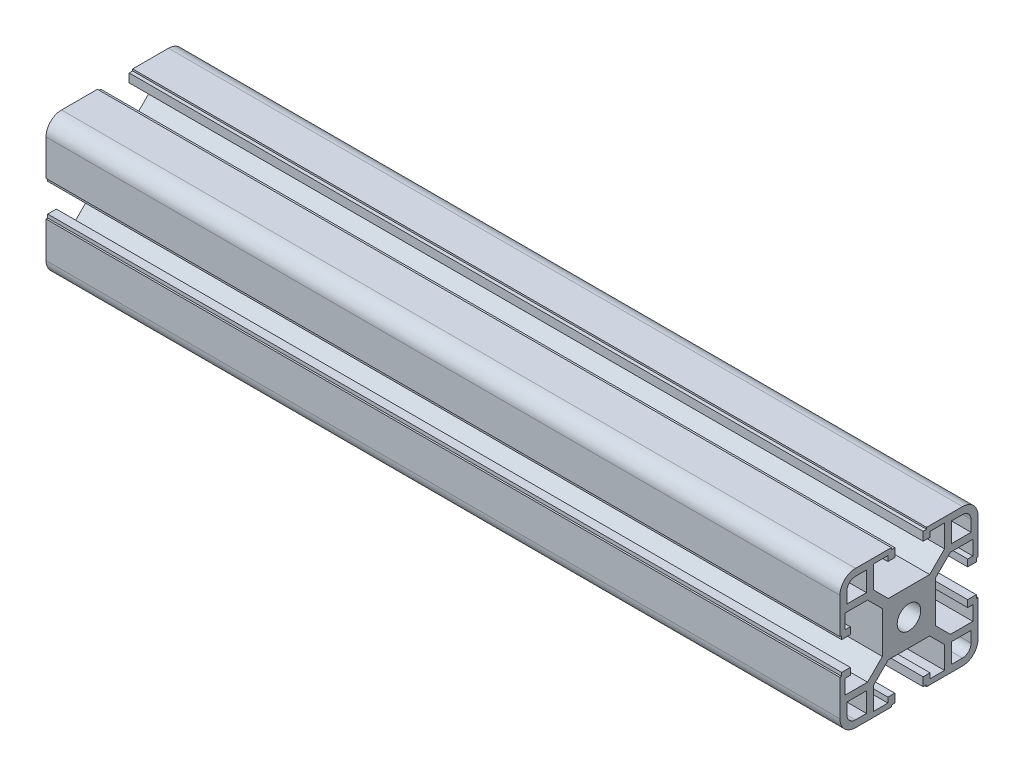
SolidWorks part; units mm, degrees
ref_plane "Front Plane" through (0, 0, 0) normal (0, 0, 1) x (1, 0, 0)
ref_plane "Top Plane" through (0, 0, 0) normal (0, 1, 0) x (1, 0, 0)
ref_plane "Right Plane" through (0, 0, 0) normal (1, 0, 0) x (0, 0, -1)
sketch "草图1" plane through (0, 0, 0) normal (0, 0, 1) x (1, 0, 0)
  line L0 (-984.975, 0) -> (-754.975, 0)
  dimension "D1" = 230
other "Aluminium profile 40 X 40B X R4.5(1)"
ref_plane "Plane1" through (-984.975, 0, 0) normal (1, 0, 0) x (0, 1, 0)
sketch "Sketch1" plane through (-984.975, 0, 0) normal (1, 0, 0) x (0, 1, 0)
  line L0 (-5.1, 20) -> (-5.1, 19.5)
  line L1 (-5.1, 19.5) -> (-4.1, 19.5)
  line L2 (-4.1, 19.5) -> (-4.1, 17)
  line L3 (-6.1, 18.5) -> (-10.3, 18.5)
  line L4 (-15.5, -20) -> (-5.1, -20)
  line L5 (-20, -15.5) -> (-20, -5.1)
  line L6 (15.5, 20) -> (5.1, 20)
  line L7 (20, 15.5) -> (20, 5.1)
  line L8 (0, 14.8756) -> (0, 0) construction
  line L9 (0, 0) -> (14.1675, 0) construction
  line L10 (-10.3, 18.5) -> (-10.3, 12)
  line L11 (-10.3, 12) -> (-6, 7.7)
  line L12 (-6, 7.7) -> (6, 7.7)
  line L13 (10.3, 12) -> (6, 7.7)
  line L14 (10.3, 18.5) -> (10.3, 12)
  line L15 (6.1, 18.5) -> (10.3, 18.5)
  line L16 (4.1, 19.5) -> (4.1, 17)
  line L17 (5.1, 19.5) -> (4.1, 19.5)
  line L18 (5.1, 20) -> (5.1, 19.5)
  line L19 (-5.1, 20) -> (-15.5, 20)
  line L20 (20, 5.1) -> (19.5, 5.1)
  line L21 (12.3, 18) -> (15.5, 18)
  line L22 (12.3, 18) -> (12.3, 12.3)
  line L23 (12.3, 12.3) -> (18, 12.3)
  line L24 (18, 15.5) -> (18, 12.3)
  line L25 (19.5, 5.1) -> (19.5, 4.1)
  line L26 (19.5, 4.1) -> (17, 4.1)
  line L27 (17, 6.1) -> (17, 4.1)
  line L28 (18.5, 6.1) -> (17, 6.1)
  line L29 (18.5, 6.1) -> (18.5, 10.3)
  line L30 (18.5, 10.3) -> (12, 10.3)
  line L31 (12, 10.3) -> (7.7, 6)
  line L32 (7.7, 6) -> (7.7, -6)
  line L33 (12, -10.3) -> (7.7, -6)
  line L34 (18.5, -10.3) -> (12, -10.3)
  line L35 (18.5, -6.1) -> (18.5, -10.3)
  line L36 (18.5, -6.1) -> (17, -6.1)
  line L37 (17, -4.1) -> (17, -6.1)
  line L38 (19.5, -4.1) -> (17, -4.1)
  line L39 (19.5, -5.1) -> (19.5, -4.1)
  line L40 (20, -5.1) -> (19.5, -5.1)
  line L41 (5.1, -20) -> (5.1, -19.5)
  line L42 (5.1, -19.5) -> (4.1, -19.5)
  line L43 (4.1, -19.5) -> (4.1, -17)
  line L44 (6.1, -17) -> (4.1, -17)
  line L45 (6.1, -18.5) -> (6.1, -17)
  line L46 (6.1, -18.5) -> (10.3, -18.5)
  line L47 (10.3, -18.5) -> (10.3, -12)
  line L48 (10.3, -12) -> (6, -7.7)
  line L49 (6, -7.7) -> (-6, -7.7)
  line L50 (-10.3, -12) -> (-6, -7.7)
  line L51 (-10.3, -18.5) -> (-10.3, -12)
  line L52 (-6.1, -18.5) -> (-10.3, -18.5)
  line L53 (-6.1, -18.5) -> (-6.1, -17)
  line L54 (-4.1, -17) -> (-6.1, -17)
  line L55 (-4.1, -19.5) -> (-4.1, -17)
  line L56 (-5.1, -19.5) -> (-4.1, -19.5)
  line L57 (-5.1, -20) -> (-5.1, -19.5)
  line L58 (-20, -5.1) -> (-19.5, -5.1)
  line L59 (5.1, -20) -> (15.5, -20)
  line L60 (-20, 5.1) -> (-20, 15.5)
  line L61 (-19.5, -5.1) -> (-19.5, -4.1)
  line L62 (-6.1, 18.5) -> (-6.1, 17)
  line L63 (-6.1, 17) -> (-4.1, 17)
  line L64 (6.1, 18.5) -> (6.1, 17)
  line L65 (4.1, 17) -> (6.1, 17)
  line L66 (-19.5, -4.1) -> (-17, -4.1)
  line L67 (-15.5, 18) -> (-12.3, 18)
  line L68 (-18, 15.5) -> (-18, 12.3)
  line L69 (-18, 12.3) -> (-12.3, 12.3)
  line L70 (-12.3, 18) -> (-12.3, 12.3)
  line L71 (-17, -6.1) -> (-17, -4.1)
  line L72 (-18.5, -6.1) -> (-17, -6.1)
  line L73 (-18.5, -6.1) -> (-18.5, -10.3)
  line L74 (-18.5, -10.3) -> (-12, -10.3)
  line L75 (-12, -10.3) -> (-7.7, -6)
  line L76 (-7.7, -6) -> (-7.7, 6)
  line L77 (-12, 10.3) -> (-7.7, 6)
  line L78 (-18.5, 10.3) -> (-12, 10.3)
  line L79 (-18.5, 6.1) -> (-18.5, 10.3)
  line L80 (-18.5, 6.1) -> (-17, 6.1)
  line L81 (-17, 4.1) -> (-17, 6.1)
  line L82 (-19.5, 4.1) -> (-17, 4.1)
  line L83 (-19.5, 5.1) -> (-19.5, 4.1)
  line L84 (-20, 5.1) -> (-19.5, 5.1)
  line L85 (20, -5.1) -> (20, -15.5)
  line L87 (-18, -12.3) -> (-12.3, -12.3)
  line L88 (-18, -12.3) -> (-18, -15.5)
  line L89 (-15.5, -18) -> (-12.3, -18)
  line L90 (-12.3, -12.3) -> (-12.3, -18)
  line L91 (12.3, -12.3) -> (18, -12.3)
  line L92 (12.3, -12.3) -> (12.3, -18)
  line L93 (12.3, -18) -> (15.5, -18)
  line L94 (18, -12.3) -> (18, -15.5)
  circle A0 centre (0, 0) radius 3.4
  arc A1 (-20, 15.5) -> (-15.5, 20) centre (-15.5, 15.5) cw
  arc A2 (20, 15.5) -> (15.5, 20) centre (15.5, 15.5) ccw
  arc A3 (-15.5, -20) -> (-20, -15.5) centre (-15.5, -15.5) cw
  arc A4 (15.5, -20) -> (20, -15.5) centre (15.5, -15.5) ccw
  arc A5 (-15.5, 18) -> (-18, 15.5) centre (-15.5, 15.5) ccw
  arc A6 (18, 15.5) -> (15.5, 18) centre (15.5, 15.5) ccw
  arc A7 (18, -15.5) -> (15.5, -18) centre (15.5, -15.5) cw
  arc A8 (-18, -15.5) -> (-15.5, -18) centre (-15.5, -15.5) ccw
  point P2 (0, 10)
  point P4 (0, 0)
  point P5 (-20, -20)
  point P6 (20, -20)
  point P7 (20, 20)
  point P8 (-20, 20)
  point P36 (-20, 20)
  point P39 (20, 20)
  point P121 (0, 0)
  dimension "D1" = 20.6
  dimension "D2" = 40
  dimension "D3" = 8.2
  dimension "D4" = 10.2
  dimension "D5" = 12.3
  dimension "D6" = 6.8
  dimension "D7" = 4.5
  dimension "D8" = 45
  dimension "D12" = 2
  dimension "D13" = 5.7
  dimension "D14" = 2
  dimension "D18" = 2.5
  dimension "D19" = 2.5
  dimension "D15" = 2.5
  dimension "D9" = 0.5
  dimension "D10" = 1.5
  dimension "D11" = 12
  dimension "D16" = 3
  dimension "D17" = 2
  dimension "D20" = 2
  dimension "D21" = 2
